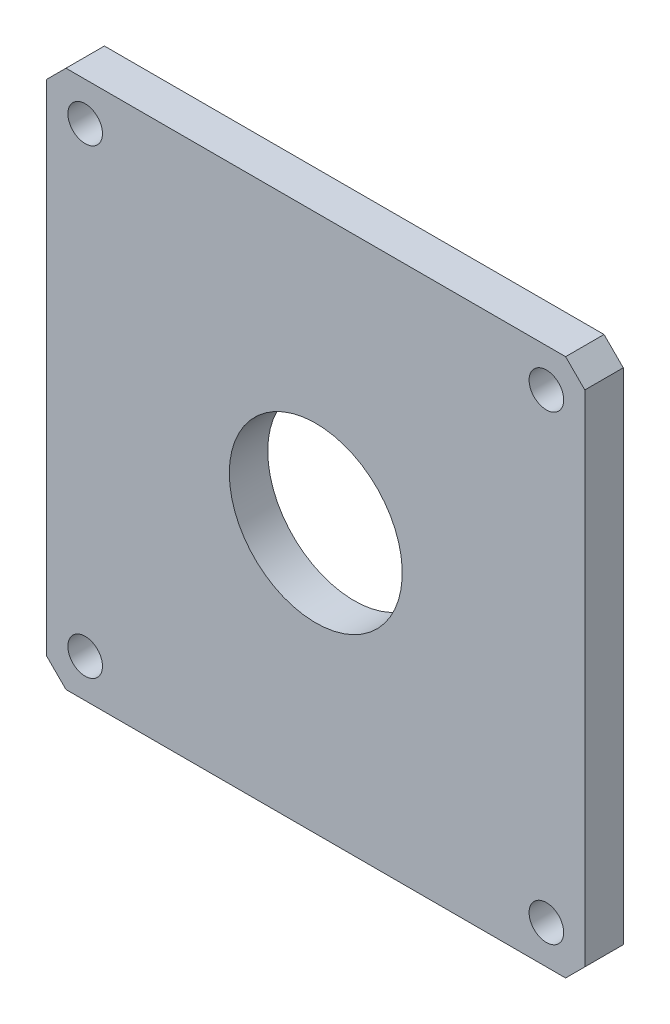
from build123d import *

# Parameters (mm, degrees)
SKETCH1_W            = 140
SKETCH1_H            = 140
BOSS_EXTRUDE1_DEPTH  = 10
CHAMFER1_SIZE        = 5
LPATTERN1_COUNT      = 2
LPATTERN1_PITCH      = 120
LPATTERN1_COUNT_DIR2 = 2
LPATTERN1_PITCH_DIR2 = 120
SKETCH4_R            = 22.5
CUT_EXTRUDE1_DEPTH   = 10


with BuildPart() as part:
    # Sketch1 → Boss-Extrude1 (new body)
    with BuildSketch(Plane.XY):
        Rectangle(SKETCH1_W, SKETCH1_H)
    extrude(amount=BOSS_EXTRUDE1_DEPTH)

    # Chamfer1
    chamfer1_edges = [part.edges().sort_by_distance(p)[0] for p in [
        (-70, 70, 5),
        (70, 70, 5),
        (70, -70, 5),
        (-70, -70, 5),
    ]]
    chamfer(chamfer1_edges, length=CHAMFER1_SIZE)

    # Sketch3 → Ø9.0 (9) Diameter Hole1 (revolve, cut)
    with BuildSketch(Plane(origin=(60, -60, 0), x_dir=(0, 1, 0), z_dir=(1, 0, 0))):
        Polygon((0, 0), (0, 22.453872786), (4.5, 19.75), (4.5, 0), align=None)
    f_9_0_9_diameter_hole1 = revolve(axis=Axis((60, -60, -6.35), (0, 0, 1)), mode=Mode.SUBTRACT)

    # LPattern1: 9.0 _9_ Diameter Hole1 2 × 2
    with Locations(*[(-j * LPATTERN1_PITCH_DIR2, i * LPATTERN1_PITCH, 0) for i in range(LPATTERN1_COUNT) for j in range(LPATTERN1_COUNT_DIR2) if (i, j) != (0, 0)]):
        add(f_9_0_9_diameter_hole1, mode=Mode.SUBTRACT)

    # Sketch4 → Cut-Extrude1 (cut)
    with BuildSketch(Plane(origin=(0, 0, 0), x_dir=(-1, 0, 0), z_dir=(0, 0, -1))):
        Circle(SKETCH4_R)
    extrude(amount=-CUT_EXTRUDE1_DEPTH, mode=Mode.SUBTRACT)


solid = part.part
